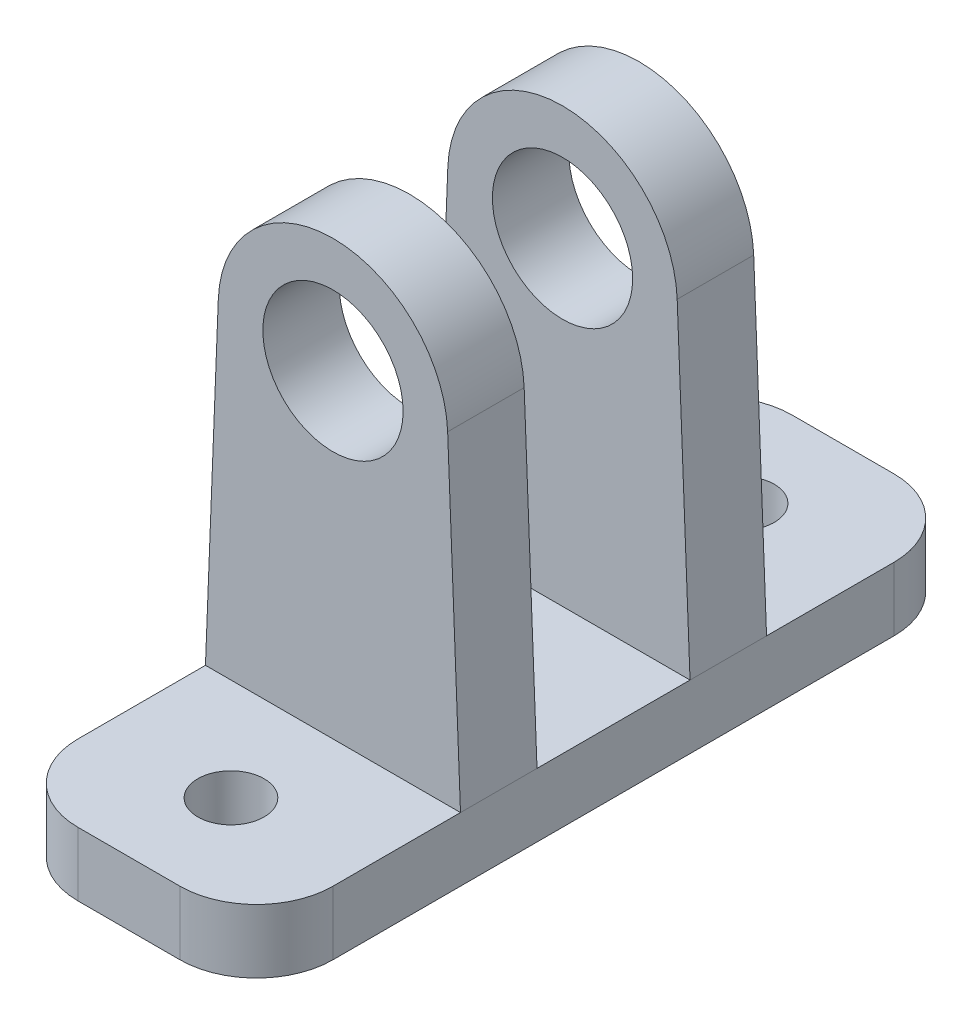
SolidWorks part; units mm, degrees
ref_plane "Front Plane" through (0, 0, 0) normal (0, 0, 1) x (1, 0, 0)
ref_plane "Top Plane" through (0, 0, 0) normal (0, 1, 0) x (1, 0, 0)
ref_plane "Right Plane" through (0, 0, 0) normal (1, 0, 0) x (0, 0, -1)
sketch "Sketch 1" plane through (0, 0, 0) normal (0, 1, 0) x (1, 0, 0)
  line L1 (-50, -60) -> (50, -60)
  line L2 (-50, -60) -> (-50, 60)
  line L3 (-50, 60) -> (50, 60)
  line L4 (50, -60) -> (50, 60)
  line L5 (-50, -60) -> (50, 60) construction
  line L6 (-50, 60) -> (50, -60) construction
  point P0 (0, 0)
  dimension "D1" = 100
  dimension "D2" = 120
extrude "Boss-Extrude 1" add sketch "Sketch 1" along normal blind 25
sketch "Sketch 2" plane through (0, 0, 60) normal (0, 0, 1) x (1, 0, 0)
  line L0 (0, -7.9075) -> (0, 168.2922) construction
  line L1 (-50, 0) -> (50, 0) construction
  line L2 (-44.9646, 151.7858) -> (-50, 25)
  line L3 (-50, 25) -> (50, 25) construction
  line L4 (-50, 25) -> (-50, 0) construction
  line L5 (-50, 25) -> (50, 25)
  line L6 (44.9646, 151.7858) -> (50, 25)
  circle A0 centre (0, 150) radius 27.5
  arc A1 (44.9646, 151.7858) -> (-44.9646, 151.7858) centre (0, 150) ccw
  point P17 (0, 25)
  dimension "D1" = 55
  dimension "D2" = 150
  dimension "D3" = 45
extrude "Boss-Extrude 2" add sketch "Sketch 2" against normal blind 30
sketch "Sketch 4" plane through (0, 0, 60) normal (0, 0, 1) x (1, 0, 0)
  line L0 (0, -12.2336) -> (0, 150.8827) construction
  line L1 (-50, 0) -> (50, 0) construction
  line L2 (-7.5, 25) -> (7.5, 25)
  line L3 (-7.5, 25) -> (-7.5, 0)
  line L4 (-7.5, 0) -> (7.5, 0)
  line L5 (7.5, 25) -> (7.5, 0)
  line L6 (-7.5, 25) -> (7.5, 0) construction
  line L7 (-7.5, 0) -> (7.5, 25) construction
  point P3 (0, 12.5)
  dimension "D1" = 25
  dimension "15" = 15
extrude "Boss-Extrude 3" add sketch "Sketch 4" along normal blind 10
mirror "Mirror 1" about plane through (0, 0, 0) normal (0, 0, 1) of "Boss-Extrude 2", "Boss-Extrude 3"
sketch "Sketch 5" plane through (0, 0, 0) normal (0, -1, 0) x (1, 0, 0)
  line L0 (-50, -60) -> (-50, 60) construction
  line L1 (50, -140) -> (-50, -140)
  line L2 (50, -140) -> (50, 140)
  line L3 (50, 140) -> (-50, 140)
  line L4 (-50, -140) -> (-50, 140)
  line L5 (50, -140) -> (-50, 140) construction
  line L6 (50, 140) -> (-50, -140) construction
  line L7 (0, -312.6276) -> (0, 307.996) construction
  line L9 (-125.9194, -100) -> (134.6035, -100) construction
  line L11 (-132.1053, 0) -> (125.2238, 0) construction
  line L13 (-44.9646, -60) -> (44.9646, -60) construction
  circle A0 centre (0, -100) radius 13
  circle A1 centre (0, 100) radius 13
  point P0 (0, 0)
  dimension "D2" = 26
  dimension "D1" = 280
extrude "Boss-Extrude 4" add sketch "Sketch 5" against normal up to surface (25 mm away) up to face at (0, 25, 0)
fillet "Fillet 1" radius 30 4 edges at (50, 12.5, 140) (-50, 12.5, 140) (50, 12.5, -140) (-50, 12.5, -140)
